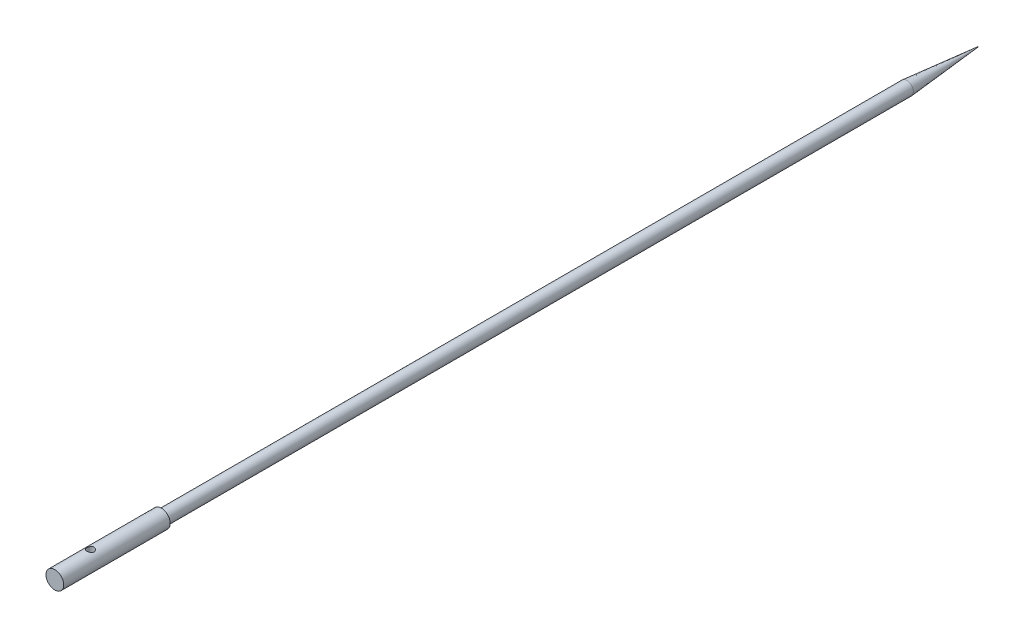
from build123d import *

# Parameters (mm, degrees)
SKETCH1_R               = 1.85
BOSS_EXTRUDE1_DEPTH     = 230
SKETCH2_R               = 2.5
BOSS_EXTRUDE2_DEPTH     = 30
CHAMFER1_SIZE           = 1.8
CHAMFER1_SIZE2          = 20
CUT_EXTRUDE1_DEPTH      = 10
CUT_EXTRUDE1_DEPTH_BACK = 10
SKETCH_3_2_R            = 1


with BuildPart() as part:
    # Sketch1 → Boss-Extrude1 (new body)
    with BuildSketch(Plane.XY):
        Circle(SKETCH1_R)
    extrude(amount=BOSS_EXTRUDE1_DEPTH)

    # Sketch2 → Boss-Extrude2 (add)
    with BuildSketch(Plane.XY.offset(230)):
        Circle(SKETCH2_R)
    extrude(amount=BOSS_EXTRUDE2_DEPTH)

    # Chamfer1
    chamfer1_edges = [part.edges().sort_by_distance(p)[0] for p in [
        (-1.85, 0, 0),
    ]]
    chamfer1_side = [part.faces().sort_by_distance(p)[0] for p in [
        (0, 0, 0),
    ]]
    chamfer(chamfer1_edges, length=CHAMFER1_SIZE, length2=CHAMFER1_SIZE2, reference=chamfer1_side[0])

    # Sketch 3_2 → Cut-Extrude1 (cut, two sides: drawn at the far end of the back side and taken through both)
    with BuildSketch(Plane(origin=(0, 0, 0), x_dir=(1, 0, 0), z_dir=(0, 1, 0)).offset(-CUT_EXTRUDE1_DEPTH_BACK)):
        with Locations(Location((0, -250, 0), (0, 0, 90))):
            Circle(SKETCH_3_2_R)
    extrude(amount=CUT_EXTRUDE1_DEPTH + CUT_EXTRUDE1_DEPTH_BACK, mode=Mode.SUBTRACT)


solid = part.part
